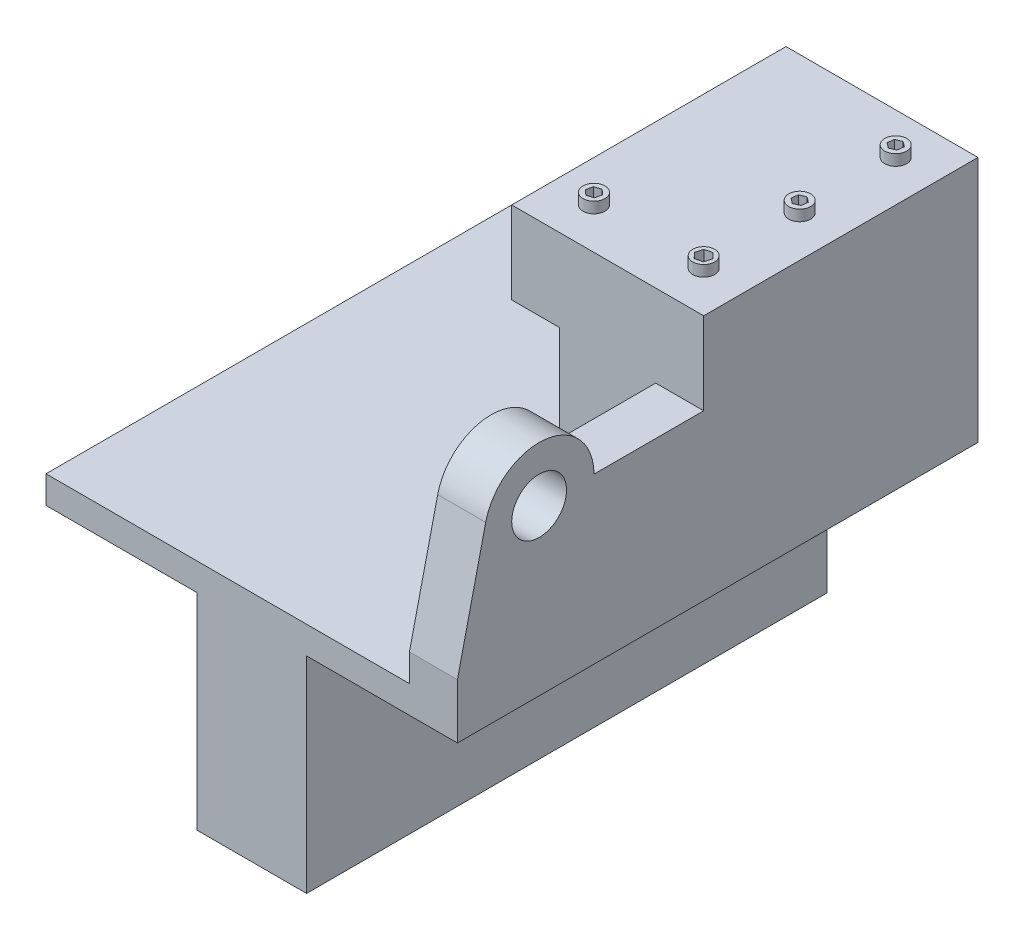
SolidWorks part; units mm, degrees
ref_plane "Front Plane" through (0, 0, 0) normal (0, 0, 1) x (1, 0, 0)
ref_plane "Top Plane" through (0, 0, 0) normal (0, 1, 0) x (1, 0, 0)
ref_plane "Right Plane" through (0, 0, 0) normal (1, 0, 0) x (0, 0, -1)
other "Configuration Table"
sketch "Sketch1" plane through (0, 0, 0) normal (0, 1, 0) x (1, 0, 0)
  line L1 (-35, 50) -> (35, 50)
  line L2 (-35, 50) -> (-35, -50)
  line L3 (-35, -50) -> (35, -50)
  line L4 (35, 50) -> (35, -50)
  line L5 (-35, 50) -> (35, -50) construction
  line L6 (-35, -50) -> (35, 50) construction
  point P0 (0, 0)
  dimension "D1" = 70
  dimension "D2" = 100
extrude "Boss-Extrude1" add sketch "Sketch1" along normal blind 30
sketch "Sketch2" plane through (0, 30, 0) normal (0, 1, 0) x (1, 0, 0)
  line L0 (20, 50) -> (20, -35) construction
  line L1 (35, 50) -> (-35, 50) construction
  line L2 (20, -35) -> (-35, -35) construction
  line L3 (-35, 50) -> (-35, -50) construction
  line L4 (35, -50) -> (35, 50) construction
  line L5 (-35, -50) -> (35, -50) construction
  line L7 (21.9131, 33.5347) -> (22.2255, 35.9241)
  line L8 (22.2255, 35.9241) -> (20.3125, 37.3894)
  line L9 (20.3125, 37.3894) -> (18.0869, 36.4653)
  line L10 (18.0869, 36.4653) -> (17.7745, 34.0759)
  line L11 (17.7745, 34.0759) -> (19.6875, 32.6106)
  line L12 (19.6875, 32.6106) -> (21.9131, 33.5347)
  line L13 (21.9131, -1.4702) -> (22.2298, 0.9217)
  line L14 (22.2298, 0.9217) -> (20.3167, 2.3919)
  line L15 (20.3167, 2.3919) -> (18.0869, 1.4702)
  line L16 (18.0869, 1.4702) -> (17.7702, -0.9217)
  line L17 (17.7702, -0.9217) -> (19.6833, -2.3919)
  line L18 (19.6833, -2.3919) -> (21.9131, -1.4702)
  line L19 (21.9131, -37.0352) -> (22.719, -34.3608)
  line L20 (22.719, -34.3608) -> (20.806, -32.3257)
  line L21 (20.806, -32.3257) -> (18.0869, -32.9648)
  line L22 (18.0869, -32.9648) -> (17.281, -35.6392)
  line L23 (17.281, -35.6392) -> (19.194, -37.6743)
  line L24 (19.194, -37.6743) -> (21.9131, -37.0352)
  line L25 (-18.1325, -36.6568) -> (-17.6315, -34.2111)
  line L26 (-17.6315, -34.2111) -> (-19.4989, -32.5543)
  line L27 (-19.4989, -32.5543) -> (-21.8675, -33.3432)
  line L28 (-21.8675, -33.3432) -> (-22.3685, -35.7889)
  line L29 (-22.3685, -35.7889) -> (-20.5011, -37.4457)
  line L30 (-20.5011, -37.4457) -> (-18.1325, -36.6568)
  circle A0 centre (-20, -35) radius 4
  circle A1 centre (20, -35) radius 4
  circle A2 centre (20, 0) radius 4
  circle A3 centre (20, 35) radius 4
  circle A4 centre (20, 35) radius 2.0869 construction
  circle A5 centre (20, 0) radius 2.0895 construction
  circle A6 centre (20, -35) radius 2.4189 construction
  circle A7 centre (-20, -35) radius 2.162 construction
  dimension "D3" = 8
  dimension "D4" = 8
  dimension "D5" = 8
  dimension "D6" = 8
  dimension "D1" = 15
  dimension "D2" = 15
  dimension "D7" = 15
  dimension "D8" = 35
  dimension "D9" = 35
extrude "Boss-Extrude2" add sketch "Sketch2" along normal blind 4
sketch "Sketch3" plane through (0, 0, 0) normal (0, -1, 0) x (1, 0, 0)
  line L0 (-35, 50) -> (35, 50) construction
  line L1 (17.5, -50) -> (-17.5, -50)
  line L2 (17.5, -50) -> (17.5, 50)
  line L3 (17.5, 50) -> (-17.5, 50)
  line L4 (-17.5, -50) -> (-17.5, 50)
  line L5 (17.5, -50) -> (-17.5, 50) construction
  line L6 (17.5, 50) -> (-17.5, -50) construction
  point P0 (0, 0)
  dimension "D1" = 35
extrude "Boss-Extrude3" add sketch "Sketch3" along normal blind 40
sketch "Sketch4" plane through (17.5, 0, 0) normal (1, 0, 0) x (0, 0, -1)
  line L0 (50, 0) -> (-50, 0) construction
  line L1 (-50, -40) -> (-139.7812, -40)
  line L2 (-139.7812, -40) -> (-129.4854, 4.5075)
  line L3 (-90, 0) -> (-50, 0)
  line L4 (-50, 0) -> (50, 0)
  line L5 (50, 0) -> (50, -40)
  line L6 (50, -40) -> (-50, -40)
  circle A0 centre (-110, 0) radius 10
  arc A1 (-90, 0) -> (-129.4854, 4.5075) centre (-110, 0) ccw
  dimension "D2" = 20
  dimension "D3" = 40
  dimension "D1" = 0
  dimension "D4" = 40
extrude "Boss-Extrude4" add sketch "Sketch4" along normal up to surface (17.5 mm away) up to face at (35, 15, 0)
sketch "Sketch5" plane through (0, -40, 0) normal (0, -1, 0) x (1, 0, 0)
  line L0 (17.5, 139.7812) -> (35, 139.7812)
  line L1 (35, 139.7812) -> (35, -50)
  line L2 (35, -50) -> (-17.5, -50)
  line L3 (-17.5, -50) -> (-17.5, 50)
  line L4 (-17.5, 50) -> (17.5, 50)
  line L5 (17.5, 50) -> (17.5, 139.7812)
extrude "Boss-Extrude5" add sketch "Sketch5" along normal blind 10
sketch "Sketch6" plane through (0, -50, 0) normal (0, -1, 0) x (1, 0, 0)
  line L0 (35, -50) -> (35, 139.7812) construction
  line L1 (35, -50) -> (-115, -50)
  line L2 (35, -50) -> (35, 139.7812)
  line L3 (35, 139.7812) -> (-115, 139.7812)
  line L4 (-115, -50) -> (-115, 139.7812)
  dimension "D1" = 150
extrude "Boss-Extrude6" add sketch "Sketch6" along normal blind 10
sketch "Sketch7" plane through (0, -60, 0) normal (0, -1, 0) x (1, 0, 0)
  line L0 (-115, 139.7812) -> (35, -50) construction
  line L1 (35, 139.7812) -> (-115, 139.7812) construction
  line L2 (-20, -50) -> (-60, -50)
  line L3 (-20, -50) -> (-20, 139.7812)
  line L4 (-20, 139.7812) -> (-60, 139.7812)
  line L5 (-60, -50) -> (-60, 139.7812)
  line L6 (-20, -50) -> (-60, 139.7812) construction
  line L7 (-20, 139.7812) -> (-60, -50) construction
  line L8 (35, -50) -> (35, 139.7812) construction
  point P4 (-40, 44.8906)
  dimension "D1" = 55
extrude "Boss-Extrude7" add sketch "Sketch7" along normal blind 75
